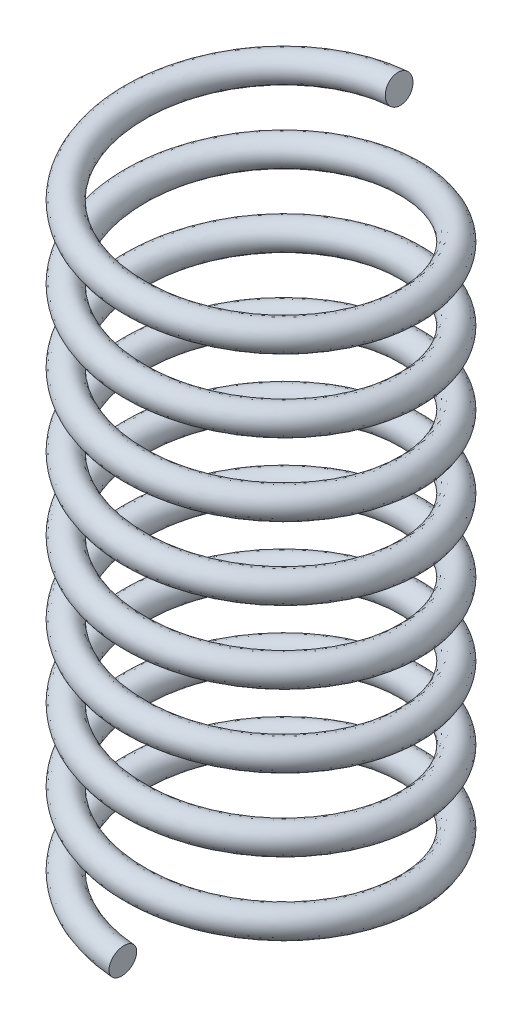
from build123d import *

# Parameters (mm, degrees)
SWEEP1_PITCH  = 6.558823529
SWEEP1_HEIGHT = 55.75
SWEEP1_RADIUS = 12.5
SKETCH2_R     = 1.25


with BuildPart() as part:
    # Sweep1: sweep along a helix
    with BuildLine() as sweep1_path:
        Helix(SWEEP1_PITCH, SWEEP1_HEIGHT, SWEEP1_RADIUS, center=(0, 0, 0), direction=(0, 1, 0), lefthand=True)
    # Sketch2 → Sweep1 (sweep)
    with BuildSketch(Plane(origin=(0, 0, 12.5), x_dir=(0, 0, 1), z_dir=(-0.9965312113765106, 0.08321985792143866, 1.3822626039964883e-14))):
        with Locations((-0.017218635, 0)):
            Circle(SKETCH2_R)
    sweep(path=sweep1_path.line, is_frenet=True)


solid = part.part
